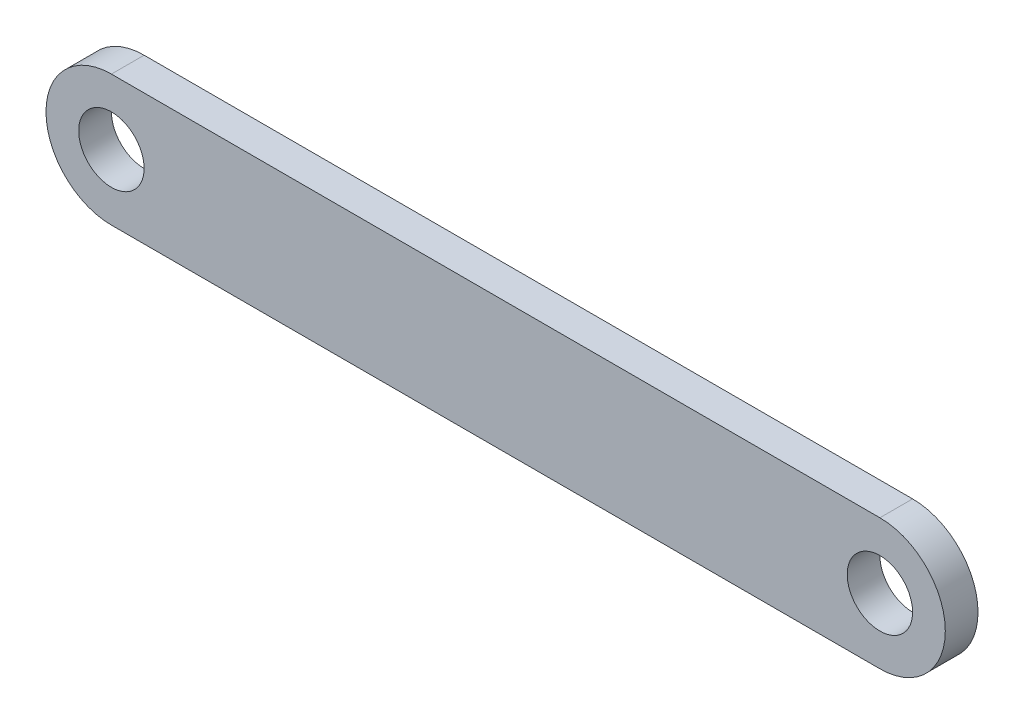
from build123d import *

# Parameters (mm, degrees)
BOSS_EXTRUDE1_DEPTH = 10
SKETCH2_R           = 10
CUT_EXTRUDE1_DEPTH  = 140.306317158


with BuildPart() as part:
    # Sketch1 → Boss-Extrude1 (new body)
    with BuildSketch(Plane.XY):
        with BuildLine():
            Line((-117.5, 20), (117.5, 20))
            ThreePointArc((117.5, 20), (137.5, 0), (117.5, -20))
            Line((117.5, -20), (-117.5, -20))
            ThreePointArc((-117.5, -20), (-137.5, 0), (-117.5, 20))
        make_face()
    extrude(amount=BOSS_EXTRUDE1_DEPTH)

    # Sketch2 → Cut-Extrude1 (cut, through all)
    with BuildSketch(Plane.XY.offset(10)):
        with Locations((-117.5, 0)):
            Circle(SKETCH2_R)
        with Locations((117.5, 0)):
            Circle(SKETCH2_R)
    extrude(amount=-CUT_EXTRUDE1_DEPTH, mode=Mode.SUBTRACT)


solid = part.part
